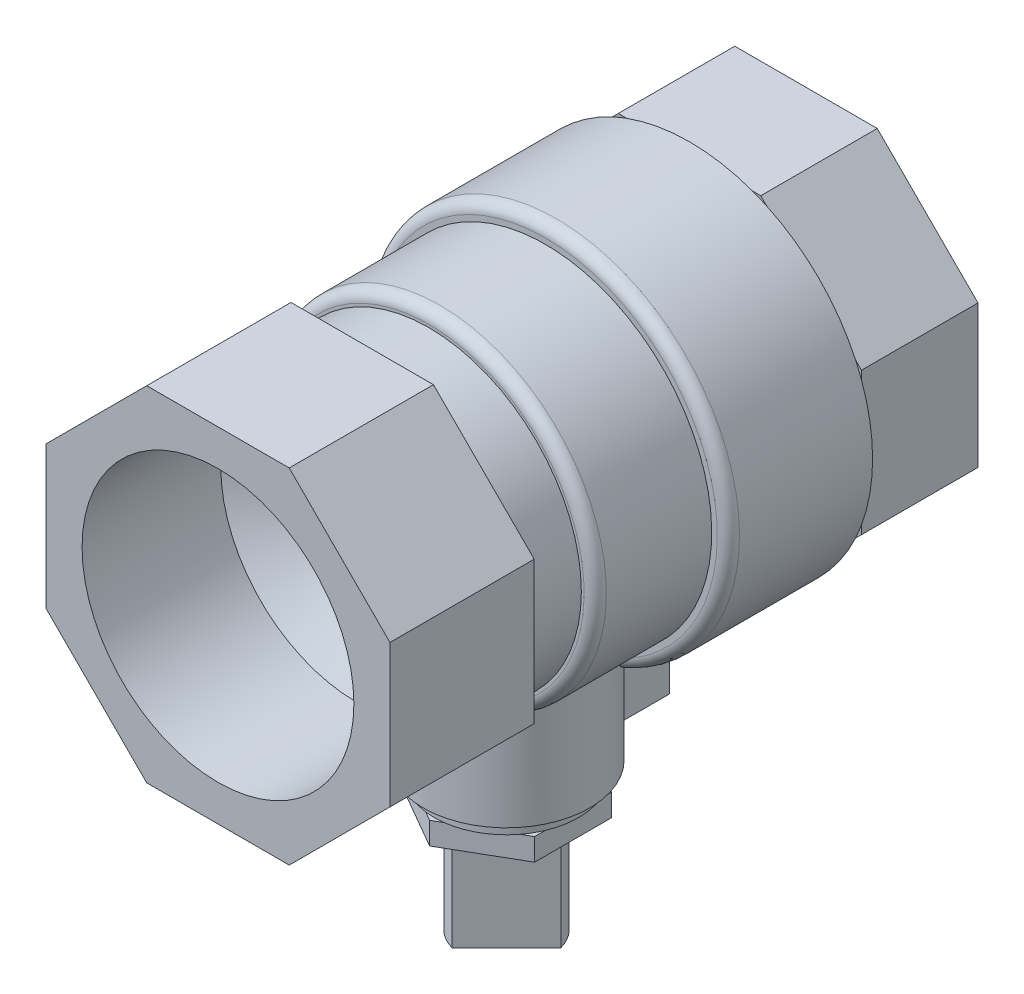
SolidWorks part; units mm, degrees
material "黄铜"
ref_plane "前视基准面" through (0, 0, 0) normal (0, 0, 1) x (1, 0, 0)
ref_plane "上视基准面" through (0, 0, 0) normal (0, 1, 0) x (1, 0, 0)
ref_plane "右视基准面" through (0, 0, 0) normal (1, 0, 0) x (0, 0, -1)
sketch "草图1" plane through (0, 0, 0) normal (0, 0, 1) x (1, 0, 0)
  circle A0 centre (0, 0) radius 15
  dimension "D1" = 30
extrude "凸台-拉伸1" add sketch "草图1" along normal blind 10.5
sketch "草图2" plane through (0, 0, 10.5) normal (0, 0, 1) x (1, 0, 0)
  circle A0 centre (0, 0) radius 13.75
  dimension "D1" = 27.5
extrude "凸台-拉伸2" add sketch "草图2" along normal blind 6
sketch "草图3" plane through (0, 0, 16.5) normal (0, 0, 1) x (1, 0, 0)
  line L0 (-1000, 0) -> (49000, 0) construction
  line L1 (6.4203, -15.5) -> (15.5, -6.4203)
  line L2 (15.5, -6.4203) -> (15.5, 6.4203)
  line L3 (15.5, 6.4203) -> (6.4203, 15.5)
  line L4 (6.4203, 15.5) -> (-6.4203, 15.5)
  line L5 (-6.4203, 15.5) -> (-15.5, 6.4203)
  line L6 (-15.5, 6.4203) -> (-15.5, -6.4203)
  line L7 (-15.5, -6.4203) -> (-6.4203, -15.5)
  line L8 (-6.4203, -15.5) -> (6.4203, -15.5)
  circle A0 centre (0, 0) radius 15.5 construction
  dimension "D1" = 31
extrude "凸台-拉伸3" add sketch "草图3" along normal blind 13
sketch "草图4" plane through (0, 0, 0) normal (0, 0, -1) x (-1, 0, 0)
  circle A0 centre (0, 0) radius 16.5
  dimension "D1" = 33
extrude "凸台-拉伸4" add sketch "草图4" along normal blind 13
sketch "草图6" plane through (0, 0, -13) normal (0, 0, -1) x (-1, 0, 0)
  line L0 (15.5, 6.4203) -> (15.5, -6.4203) construction
  line L1 (15.5, -6.4203) -> (15.5, 6.4203)
  line L2 (15.5, 6.4203) -> (6.4203, 15.5)
  line L3 (6.4203, 15.5) -> (-6.4203, 15.5)
  line L4 (-6.4203, 15.5) -> (-15.5, 6.4203)
  line L5 (-15.5, 6.4203) -> (-15.5, -6.4203)
  line L6 (-15.5, -6.4203) -> (-6.4203, -15.5)
  line L7 (-6.4203, -15.5) -> (6.4203, -15.5)
  line L8 (6.4203, -15.5) -> (15.5, -6.4203)
  circle A0 centre (0, 0) radius 15.5 construction
  dimension "D1" = 31
extrude "凸台-拉伸5" add sketch "草图6" along normal offset from surface (10.5 mm away) 53 up to face at (0, 0, 29.5)
fillet "圆角1" radius 1 2 edges at (15, 0, 10.5) (-16.5, 0, 0)
sketch "草图7" plane through (0, 0, 29.5) normal (0, 0, 1) x (1, 0, 0)
  circle A0 centre (0, 0) radius 5
  dimension "D1" = 10
hole_wizard "G3/4 螺纹孔1" positions "3D草图1" profile "草图8" tap size "G3/4" standard "GB"
sketch3d "3D草图1"
  point P0 (0, 0, 29.5)
sketch "草图8" plane through (0, 0, 29.5) normal (1, 0, 0) x (0, -1, 0)
  line L0 (0, 0) -> (0, 19.8605)
  line L1 (0, 19.8605) -> (12.25, 12.5)
  line L2 (12.25, 12.5) -> (12.25, 0)
  line L5 (12.25, 0) -> (0, 0)
  line L10 (0, 19.8605) -> (-12.25, 12.5) construction
  line L11 (0, -6.35) -> (0, 107.95) construction
  dimension "螺纹孔钻头直径" = 24.5
  dimension "螺纹孔钻头深度" = 12.5
  dimension "导头角度" = 118
cosmetic thread "孔螺蚊线1" parameters "D1"=12.5, "D2"=26.441
hole_wizard "G3/4 螺纹孔2" positions "草图9" profile "草图10" tap size "G3/4" standard "GB"
sketch "草图9" plane through (0, 0, -23.5) normal (0, 0, -1) x (-1, 0, 0)
  point P0 (0, 0)
sketch "草图10" plane through (0, 0, -23.5) normal (1, 0, 0) x (0, 1, 0)
  line L0 (0, 0) -> (0, 19.8605)
  line L1 (0, 19.8605) -> (12.25, 12.5)
  line L2 (12.25, 12.5) -> (12.25, 0)
  line L5 (12.25, 0) -> (0, 0)
  line L10 (0, 19.8605) -> (-12.25, 12.5) construction
  line L11 (0, -6.35) -> (0, 107.95) construction
  dimension "螺纹孔钻头直径" = 24.5
  dimension "螺纹孔钻头深度" = 12.5
  dimension "导头角度" = 118
cosmetic thread "孔螺蚊线2" parameters "D1"=12.5, "D2"=26.441
sketch "草图11" plane through (0, 0, -23.5) normal (0, 0, -1) x (-1, 0, 0)
  circle A0 centre (0, 0) radius 7.5
  dimension "D1" = 15
extrude "切除-拉伸1" cut sketch "草图11" against normal up to next
ref_plane "基准面1" through (0, -16.5, 0) normal (0, -1, 0) x (-1, 0, 0)
ref_plane "基准面2" through (0, -23.5, 0) normal (0, -1, 0) x (-1, 0, 0)
sketch "草图12" plane through (0, -23.5, 0) normal (0, -1, 0) x (-1, 0, 0)
  line L0 (0, -1000) -> (0, 49000) construction
  line L1 (6.4203, 23.5) -> (-6.4203, 23.5) construction
  line L2 (-1000.0119, -11) -> (48999.9881, -11) construction
  line L5 (-2.2, 9) -> (2.2, 9)
  line L9 (-2.2, 3.6701) -> (-2.2, 9)
  line L10 (2.2, 3.6701) -> (2.2, 9)
  arc A0 (-2.2, 3.6701) -> (2.2, 3.6701) centre (0, -3.5) ccw
  dimension "D2" = 15
  dimension "D1" = 27
  dimension "D3" = 20
  dimension "D4" = 4.4
extrude "凸台-拉伸6" add sketch "草图12" against normal up to next
sketch "草图13" plane through (0, -23.5, 0) normal (0, -1, 0) x (1, 0, 0)
  circle A0 centre (0, 3.5) radius 6.5
  arc A1 (2.2, -3.6701) -> (-2.2, -3.6701) centre (0, 3.5) ccw construction
  dimension "D1" = 1
extrude "凸台-拉伸7" add sketch "草图13" along normal blind 1.25
sketch "草图14" plane through (0, -24.75, 0) normal (0, -1, 0) x (1, 0, 0)
  line L0 (-1000, 3.5) -> (49000, 3.5) construction
  line L1 (6, 6.9641) -> (0, 10.4282)
  line L2 (0, 10.4282) -> (-6, 6.9641)
  line L3 (-6, 6.9641) -> (-6, 0.0359)
  line L4 (-6, 0.0359) -> (0, -3.4282)
  line L5 (0, -3.4282) -> (6, 0.0359)
  line L6 (6, 0.0359) -> (6, 6.9641)
  line L7 (0, -996.5) -> (0, 49003.5) construction
  circle A0 centre (0, 3.5) radius 6 construction
  dimension "D1" = 12
extrude "凸台-拉伸8" add sketch "草图14" along normal blind 2
sketch "草图15" plane through (0, -26.75, 0) normal (0, -1, 0) x (1, 0, 0)
  circle A0 centre (0, 3.5) radius 4
  dimension "D1" = 8
extrude "凸台-拉伸9" add sketch "草图15" along normal blind 10
sketch "草图16" plane through (0, -36.75, 0) normal (0, -1, 0) x (1, 0, 0)
  line L0 (0, 3.5) -> (35355.3391, -35351.8391) construction
  line L1 (-1000, 3.5) -> (49000, 3.5) construction
  line L2 (-3.8637, 4.5353) -> (1.0353, -0.3637)
  line L3 (-1.0353, 7.3637) -> (3.8637, 2.4647)
  arc A0 (3.8637, 2.4647) -> (-1.0353, 7.3637) centre (0, 3.5) ccw
  circle A1 centre (0, 3.5) radius 4
  arc A2 (-3.8637, 4.5353) -> (1.0353, -0.3637) centre (0, 3.5) ccw
  dimension "D1" = 45
  dimension "D2" = 4
  dimension "D3" = 0
extrude "切除-拉伸2" cut sketch "草图16" against normal up to surface (10 mm away) up to face at (4, -26.75, 3.5)
